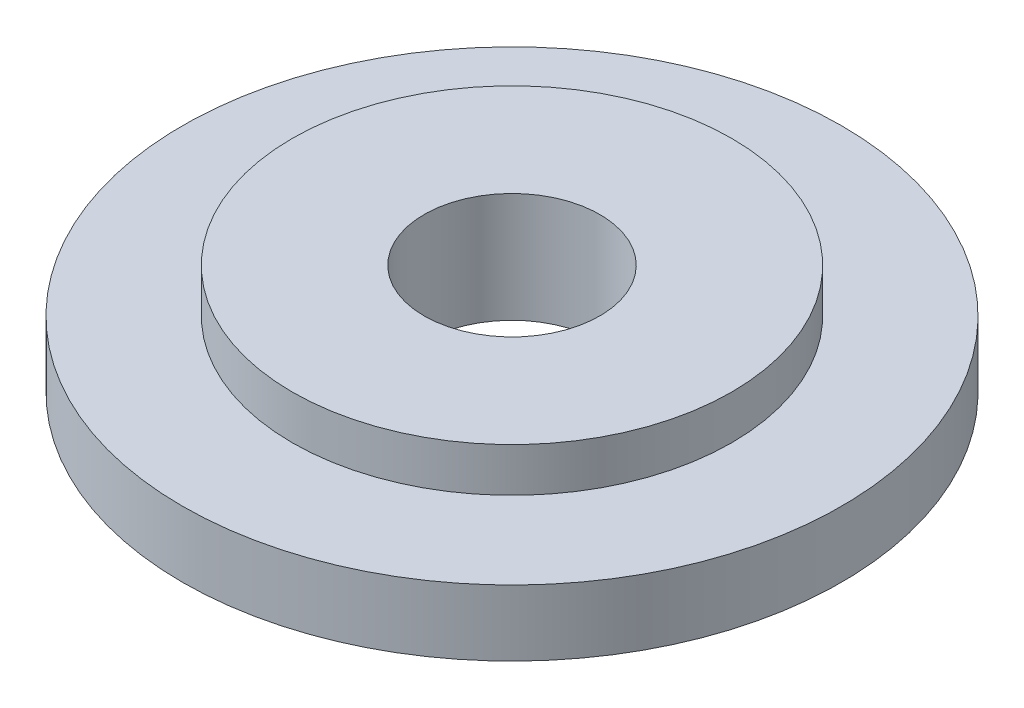
SolidWorks part; units mm, degrees
ref_plane "前视基准面" through (0, 0, 0) normal (0, 0, 1) x (1, 0, 0)
ref_plane "上视基准面" through (0, 0, 0) normal (0, 1, 0) x (1, 0, 0)
ref_plane "右视基准面" through (0, 0, 0) normal (1, 0, 0) x (0, 0, -1)
sketch "草图1" plane through (0, 0, 0) normal (0, 1, 0) x (1, 0, 0)
  circle A0 centre (0, 0) radius 15
extrude "凸台-拉伸1" add sketch "草图1" along normal blind 3
sketch "草图2" plane through (0, 3, 0) normal (0, 1, 0) x (1, 0, 0)
  circle A0 centre (0, 0) radius 10
extrude "凸台-拉伸2" add sketch "草图2" along normal blind 2
sketch "草图3" plane through (0, 5, 0) normal (0, 1, 0) x (1, 0, 0)
  circle A0 centre (0, 0) radius 4
extrude "切除-拉伸1" cut sketch "草图3" against normal through all
